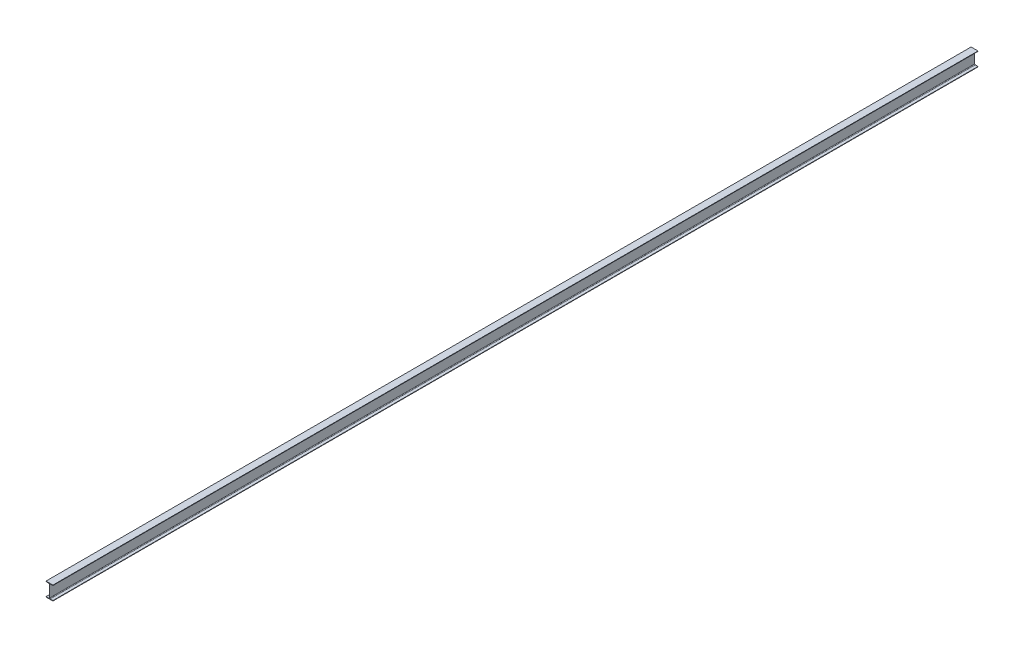
SolidWorks part; units mm, degrees
ref_plane "Front Plane" through (0, 0, 0) normal (0, 0, 1) x (1, 0, 0)
ref_plane "Top Plane" through (0, 0, 0) normal (0, 1, 0) x (1, 0, 0)
ref_plane "Right Plane" through (0, 0, 0) normal (1, 0, 0) x (0, 0, -1)
other "Configuration Table"
sketch "Sketch1" plane through (0, 0, 0) normal (0, 0, 1) x (1, 0, 0)
  line L0 (0, 0) -> (0, 300) construction
  line L1 (75, 0) -> (-75, 0)
  line L2 (-75, 0) -> (-75, 9)
  line L3 (-75, 9) -> (-16.25, 9)
  line L4 (3.25, 22) -> (3.25, 278)
  line L6 (-75, 291) -> (-75, 300)
  line L7 (-75, 300) -> (75, 300)
  line L8 (-3.25, 22) -> (-3.25, 278)
  line L9 (75, 291) -> (75, 300)
  line L10 (16.25, 291) -> (75, 291)
  line L11 (75, 9) -> (16.25, 9)
  line L12 (75, 0) -> (75, 9)
  line L13 (-16.25, 291) -> (-75, 291)
  arc A0 (16.25, 9) -> (3.25, 22) centre (16.25, 22) cw
  arc A1 (-3.25, 22) -> (-16.25, 9) centre (-16.25, 22) cw
  arc A2 (3.25, 278) -> (16.25, 291) centre (16.25, 278) cw
  arc A3 (-3.25, 278) -> (-16.25, 291) centre (-16.25, 278) ccw
  point P18 (3.25, 9)
  point P21 (-3.25, 9)
  point P24 (3.25, 291)
  point P27 (-3.25, 291)
  dimension "D6" = 13
  dimension "D1" = 300
  dimension "D2" = 150
  dimension "D3" = 6.5
  dimension "D4" = 9
  dimension "D5" = 9
extrude "Boss-Extrude1" add sketch "Sketch1" along normal blind 20067
